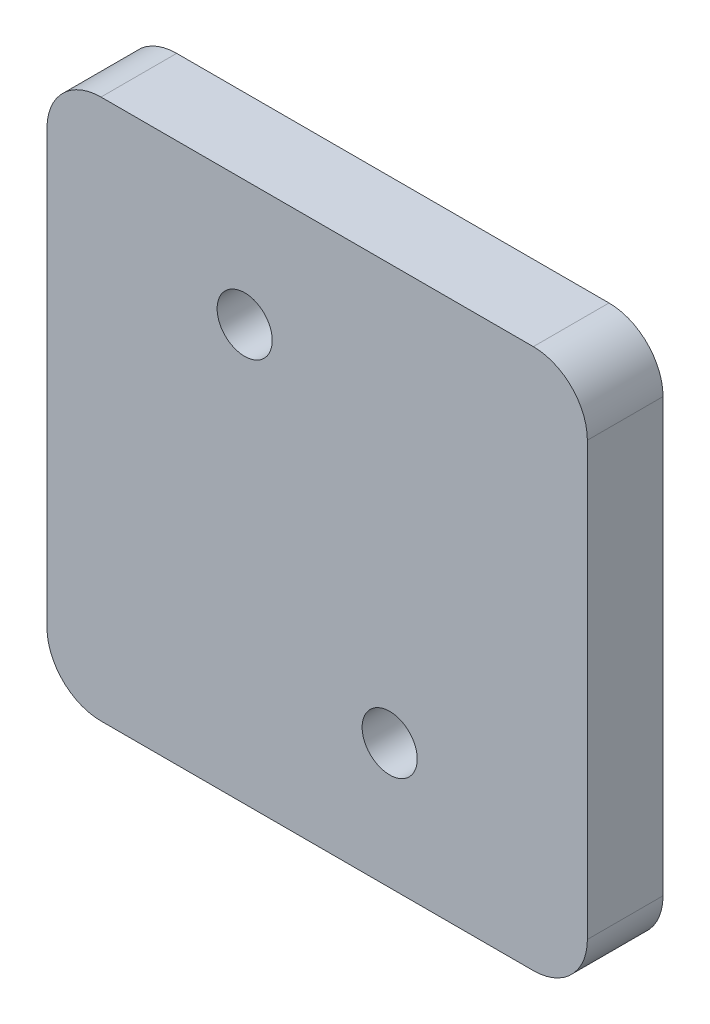
SolidWorks part; units mm, degrees
material "普通碳钢"
ref_plane "前视基准面" through (0, 0, 0) normal (0, 0, 1) x (1, 0, 0)
ref_plane "上视基准面" through (0, 0, 0) normal (0, 1, 0) x (1, 0, 0)
ref_plane "右视基准面" through (0, 0, 0) normal (1, 0, 0) x (0, 0, -1)
sketch "草图1" plane through (0, 0, 0) normal (0, 0, 1) x (1, 0, 0)
  line L0 (-40, -50) -> (40, -50) construction
  line L1 (-50, 50) -> (50, 50)
  line L2 (-50, 50) -> (-50, -50)
  line L3 (-50, -50) -> (50, -50)
  line L4 (50, 50) -> (50, -50)
  line L5 (50, -40) -> (50, 40) construction
  line L6 (-50, 40) -> (-50, -40) construction
  dimension "D1" = 100
extrude "凸台-拉伸1" add sketch "草图1" along normal blind 14 contours L2 L3 L4 L1
hole_wizard "M12 螺纹孔1" positions "3D草图2" profile "草图2" tap size "M12" standard "GB" end condition through all
sketch3d "3D草图2"
  line L0 (-35.7771, 15.6525, 14) -> (8.9443, 38.0132, 14) construction
  line L2 (8.9443, 38.0132, 14) -> (35.7771, -15.6525, 14) construction
  line L3 (35.7771, -15.6525, 14) -> (-8.9443, -38.0132, 14) construction
  line L4 (-8.9443, -38.0132, 14) -> (-35.7771, 15.6525, 14) construction
  line L9 (-25, 50, 14) -> (25, -50, 14) construction
  line L10 (-50, 50, 14) -> (50, 50, 14) construction
  line L11 (-50, -50, 14) -> (50, -50, 14) construction
  line L13 (-50, 50, 14) -> (-50, -50, 14) construction
  line L14 (-35.7771, 15.6525, 14) -> (35.7771, -15.6525, 14) construction
  point P53 (0, 0, 14)
  point P54 (0, 0, 14)
  point P55 (-13.4164, 26.8328, 14)
  point P57 (13.4164, -26.8328, 14)
  point P61 (-13.4164, 26.8328, 14)
  point P63 (13.4164, -26.8328, 14)
  dimension "D1" = 50
  dimension "D2" = 60
  dimension "D3" = 25
  dimension "D4" = 25
sketch "草图2" plane through (13.4164, -26.8328, 14) normal (1, 0, 0) x (0, -1, 0)
  line L0 (0, 0) -> (0, 14)
  line L1 (0, 14) -> (5.1, 14)
  line L2 (5.1, 14) -> (5.1, 0)
  line L5 (5.1, 0) -> (0, 0)
  line L11 (0, -6.35) -> (0, 107.95) construction
  dimension "通孔螺纹孔钻头直径" = 10.2
  dimension "通孔螺纹孔钻头深度" = 14
cosmetic thread "孔螺蚊线5"
cosmetic thread "孔螺蚊线6"
fillet "圆角1" radius 10 4 edges at (50, 50, 7) (-50, 50, 7) (50, -50, 7) (-50, -50, 7)
